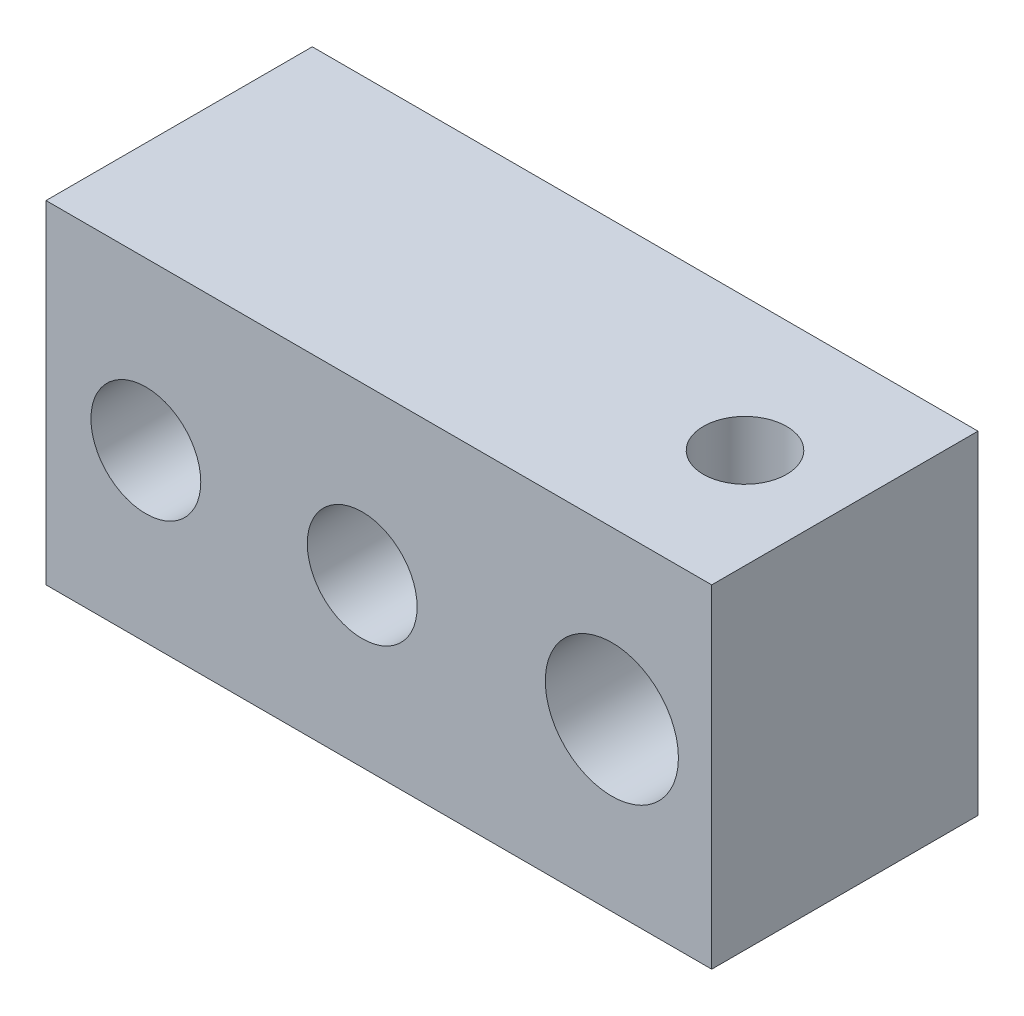
SolidWorks part; units mm, degrees
material "6061铝"
ref_plane "前视基准面" through (0, 0, 0) normal (0, 0, 1) x (1, 0, 0)
ref_plane "上视基准面" through (0, 0, 0) normal (0, 1, 0) x (1, 0, 0)
ref_plane "右视基准面" through (0, 0, 0) normal (1, 0, 0) x (0, 0, -1)
sketch "草图1" plane through (0, 0, 0) normal (0, 0, 1) x (1, 0, 0)
  line L1 (-10, 5) -> (10, 5)
  line L2 (-10, 5) -> (-10, -5)
  line L3 (-10, -5) -> (10, -5)
  line L4 (10, 5) -> (10, -5)
  line L5 (-10, 5) -> (10, -5) construction
  line L6 (-10, -5) -> (10, 5) construction
  circle A0 centre (0, 0) radius 2
  dimension "D1" = 4
  dimension "D2" = 10
  dimension "D3" = 20
extrude "凸台-拉伸1" add sketch "草图1" along normal blind 8
sketch "草图2" plane through (0, 0, 0) normal (0, 0, -1) x (-1, 0, 0)
  line L0 (-10, -5) -> (-10, 5) construction
  line L1 (-12.7582, 10.3246) -> (-3, 10.3246)
  line L2 (-12.7582, 10.3246) -> (-12.7582, -5.8474)
  line L3 (-12.7582, -5.8474) -> (-3, -5.8474)
  line L4 (-3, 10.3246) -> (-3, -5.8474)
  dimension "D1" = 7
extrude "切除-拉伸1" cut sketch "草图2" against normal blind 22
other "移动面1" face at (-10, 0, 4) parameters "D1"=7
hole_wizard "Ø3.3 (3.3) 直径孔1" positions "草图3" profile "草图5" hole size "Ø3.3" standard "GB"
sketch "草图3" plane through (0, 0, 0) normal (0, 0, -1) x (-1, 0, 0)
  line L0 (17, 5) -> (17, -5) construction
  point P0 (7.5, 0)
  point P2 (14, 0)
  dimension "D1" = 3
  dimension "D2" = 6.5
sketch "草图5" plane through (-7.5, 0, 0) normal (1, 0, 0) x (0, 1, 0)
  line L0 (0, 0) -> (0, 12.4914)
  line L1 (0, 12.4914) -> (1.65, 11.5)
  line L2 (1.65, 11.5) -> (1.65, 0)
  line L5 (1.65, 0) -> (0, 0)
  line L10 (0, 12.4914) -> (-1.65, 11.5) construction
  line L11 (0, -6.35) -> (0, 107.95) construction
  dimension "孔直径" = 3.3
  dimension "孔深度" = 11.5
  dimension "导头角度" = 118
hole_wizard "M3 螺纹孔1" positions "草图6" profile "草图7" tap size "M3" standard "GB" end condition through all
sketch "草图6" plane through (0, 5, 0) normal (0, 1, 0) x (1, 0, 0)
  line L0 (3, -8) -> (3, 0) construction
  point P0 (0, -4)
  dimension "D1" = 4
  dimension "D2" = 3
cosmetic thread "孔螺蚊线1" parameters "D2"=3
sketch "草图7" plane through (0, 5, 4) normal (1, 0, 0) x (0, 0, 1)
  line L0 (0, 0) -> (0, 10)
  line L1 (0, 10) -> (1.25, 10)
  line L2 (1.25, 10) -> (1.25, 0)
  line L5 (1.25, 0) -> (0, 0)
  line L11 (0, -6.35) -> (0, 107.95) construction
  dimension "通孔螺纹孔钻头直径" = 2.5
  dimension "通孔螺纹孔钻头深度" = 10
